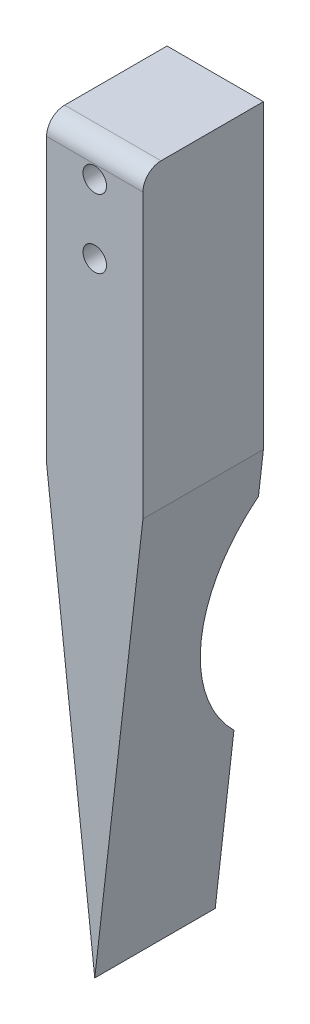
from build123d import *

# Parameters (mm, degrees)
EXTRUDE_1_DEPTH          = 10
SKETCH_3_R               = 0.975
CUT_EXTRUDE_2_DEPTH      = 61.959002617
FILLET_1_R               = 1.5
CUT_EXTRUDE_3_DEPTH      = 62.351446601
CUT_EXTRUDE_3_DEPTH_BACK = 62.351446601
SKETCH_6_R               = 12.5


with BuildPart() as part:
    # 草图1 → 凸台-拉伸1 (new body)
    with BuildSketch(Plane.XY):
        Polygon((-4, 0), (4, 0), (4, -25), (0, -60), (-4, -25), align=None)
    extrude(amount=EXTRUDE_1_DEPTH)

    # 草图3 → 切除-拉伸2 (cut, through all)
    with BuildSketch(Plane.XY.offset(10)):
        with Locations((0, -8.284315822)):
            Circle(SKETCH_3_R)
        with Locations((0, -2.584315822)):
            Circle(SKETCH_3_R)
    extrude(amount=-CUT_EXTRUDE_2_DEPTH, mode=Mode.SUBTRACT)

    # 圆角1
    fillet_1_edges = [part.edges().sort_by_distance(p)[0] for p in [
        (0, 0, 10),
    ]]
    fillet(fillet_1_edges, radius=FILLET_1_R)

    # 草图6 → 切除-拉伸3 (cut, two sides: drawn at the far end of the back side and taken through both)
    with BuildSketch(Plane.ZY.offset(4).offset(-CUT_EXTRUDE_3_DEPTH_BACK)):
        with Locations((-8.77, -37.5)):
            Circle(SKETCH_6_R)
    extrude(amount=CUT_EXTRUDE_3_DEPTH + CUT_EXTRUDE_3_DEPTH_BACK, mode=Mode.SUBTRACT)


solid = part.part
